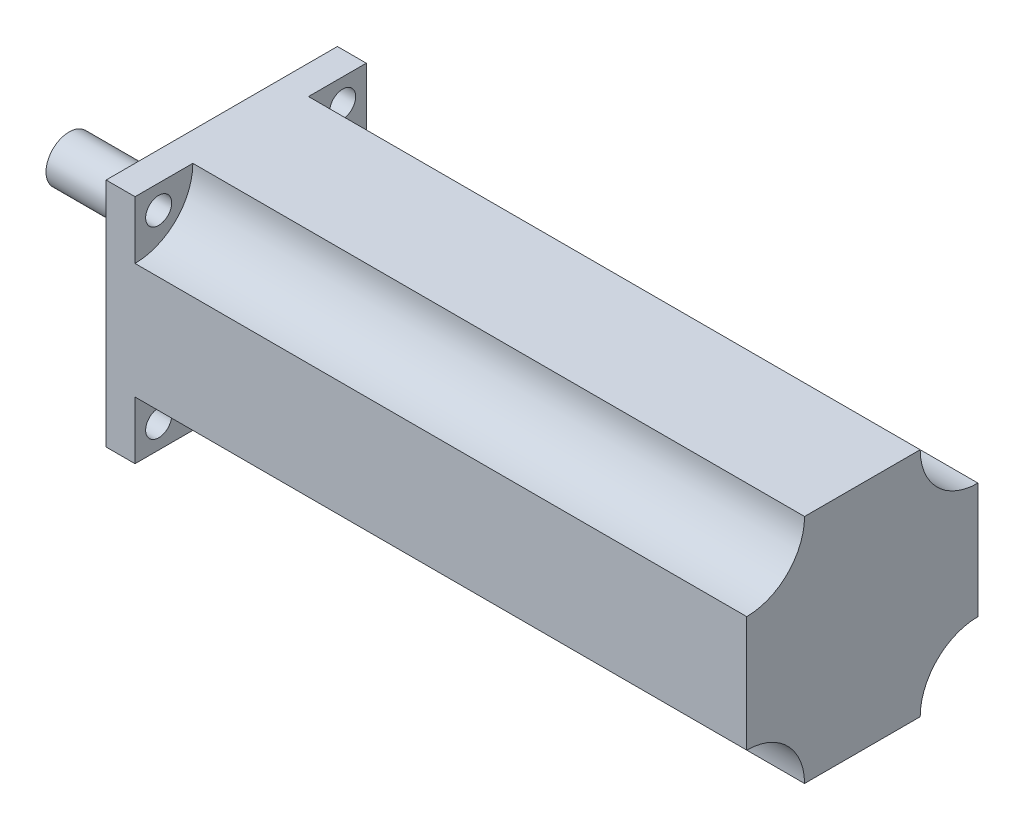
from build123d import *

# Parameters (mm, degrees)
SKETCH1_W           = 110.8
SKETCH1_H           = 40
BOSS_EXTRUDE1_DEPTH = 40
SKETCH2_R           = 15
BOSS_EXTRUDE2_DEPTH = 2.6
SKETCH3_R           = 4
BOSS_EXTRUDE3_DEPTH = 23.8
SKETCH4_R           = 10
CUT_EXTRUDE1_DEPTH  = 105.8
CIRPATTERN1_COUNT   = 4


with BuildPart() as part:
    # Sketch1 → Boss-Extrude1 (new body)
    with BuildSketch(Plane.XY):
        Rectangle(SKETCH1_W, SKETCH1_H)
    extrude(amount=BOSS_EXTRUDE1_DEPTH)

    # Sketch2 → Boss-Extrude2 (add)
    with BuildSketch(Plane.ZY.offset(55.4)):
        with Locations(Location((20, 0, 0), (0, 0, 90))):
            Circle(SKETCH2_R)
    extrude(amount=BOSS_EXTRUDE2_DEPTH)

    # Sketch3 → Boss-Extrude3 (add)
    with BuildSketch(Plane.ZY.offset(58)):
        with Locations(Location((20, 0, 0), (0, 0, 270))):
            Circle(SKETCH3_R)
    extrude(amount=BOSS_EXTRUDE3_DEPTH)

    # Sketch4 → Cut-Extrude1 (cut)
    with BuildSketch(Plane(origin=(55.4, 0, 0), x_dir=(0, 0, -1), z_dir=(1, 0, 0))):
        with Locations((-40, 20)):
            Circle(SKETCH4_R)
        with Locations((0, 20)):
            Circle(SKETCH4_R)
        with Locations((-40, -20)):
            Circle(SKETCH4_R)
        with Locations((0, -20)):
            Circle(SKETCH4_R)
    extrude(amount=-CUT_EXTRUDE1_DEPTH, mode=Mode.SUBTRACT)

    # Sketch5 → M4 Clearance Hole1 (revolve, cut)
    with BuildSketch(Plane(origin=(-55.4, 15.909902577, 4.090097423), x_dir=(0, 0, 1), z_dir=(0, 1, 0))):
        Polygon((0, 0), (0, 258.851936393), (2.25, 257.5), (2.25, 0), align=None)
    m4_clearance_hole1 = revolve(axis=Axis((-61.75, 15.909902577, 4.090097423), (1, 0, 0)), mode=Mode.SUBTRACT)

    # CirPattern1: M4 Clearance Hole1 ×4 about axis
    cirpattern1_axis = Axis((0, 0, 20), (1, 0, 0))
    for i in range(1, CIRPATTERN1_COUNT):
        add(m4_clearance_hole1.rotate(cirpattern1_axis, i * 360 / CIRPATTERN1_COUNT), mode=Mode.SUBTRACT)


solid = part.part
